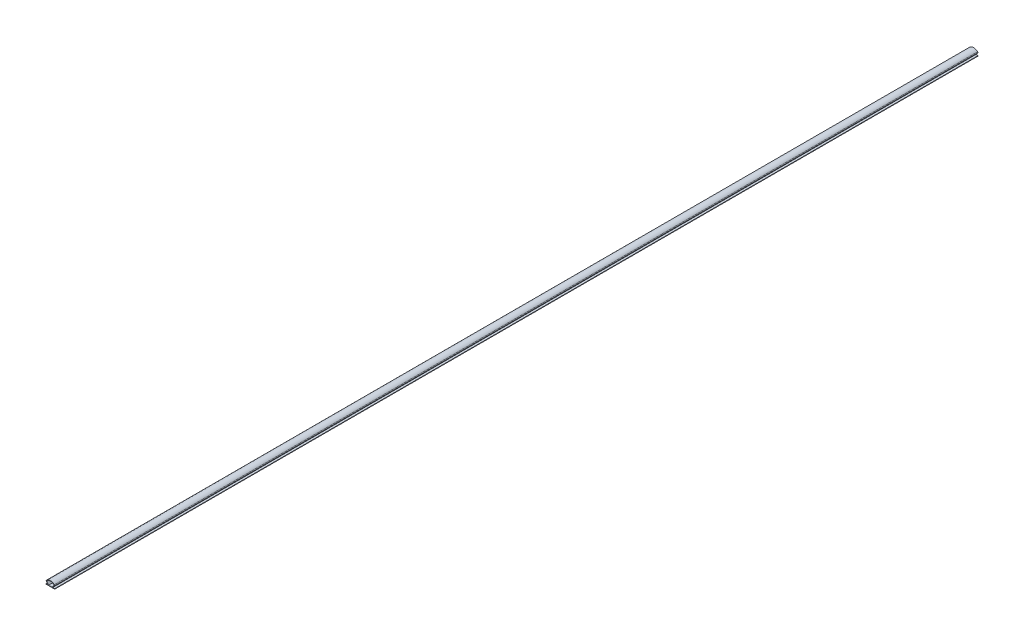
SolidWorks part; units mm, degrees
ref_plane "前视" through (0, 0, 0) normal (0, 0, 1) x (1, 0, 0)
ref_plane "上视" through (0, 0, 0) normal (0, 1, 0) x (1, 0, 0)
ref_plane "右视" through (0, 0, 0) normal (1, 0, 0) x (0, 0, -1)
sketch "草图1" plane through (0, 0, 0) normal (0, 0, 1) x (1, 0, 0)
  line L0 (0, 0) -> (0, 22.9077) construction
  line L1 (-4.5569, 4.1381) -> (-2.6457, 1.7989)
  line L2 (-2.6457, 1.7989) -> (-5, 1.7989)
  line L3 (-2, 1.7989) -> (2, 1.7989)
  line L4 (4.5569, 4.1381) -> (2.6457, 1.7989)
  line L5 (1.5915, 1.2989) -> (-5, 1.2989)
  line L6 (-4.1697, 4.4545) -> (-2, 1.7989)
  line L7 (4.1697, 4.4545) -> (2, 1.7989)
  line L8 (1.5915, 1.2989) -> (5, 1.2989)
  line L9 (-5, 1.7989) -> (-5, 1.2989)
  line L10 (5, 1.7989) -> (5, 1.2989)
  line L11 (2.6457, 1.7989) -> (5, 1.7989) construction
  line L12 (-1.5915, 1.2989) -> (-5, 1.2989) construction
  line L13 (-4.1697, 4.4545) -> (-1.5915, 1.2989) construction
  line L14 (4.1697, 4.4545) -> (1.5915, 1.2989) construction
  line L15 (2.6457, 1.7989) -> (5, 1.7989)
  arc A0 (-4.4771, 5.4902) -> (4.4771, 5.4902) centre (0, 0.8534) cw
  arc A1 (4.4771, 5.4902) -> (4.5569, 4.1381) centre (3.7825, 4.7708) cw
  arc A2 (-4.4771, 5.4902) -> (-4.5569, 4.1381) centre (-3.7825, 4.7708) ccw
  arc A3 (-4.1298, 5.1305) -> (-4.1697, 4.4545) centre (-3.7825, 4.7708) ccw
  arc A4 (-4.1298, 5.1305) -> (4.1298, 5.1305) centre (0, 0.8534) cw
  arc A5 (4.1298, 5.1305) -> (4.1697, 4.4545) centre (3.7825, 4.7708) cw
  point P12 (5.0968, 4.7989)
  point P15 (-5.0968, 4.7989)
  dimension "D4" = 1
  dimension "D1" = 10
  dimension "D2" = 5.5
  dimension "D3" = 3
  dimension "D6" = 4
  dimension "D5" = 0.5
extrude "凸台-拉伸1" add sketch "草图1" along normal mid plane 1058
